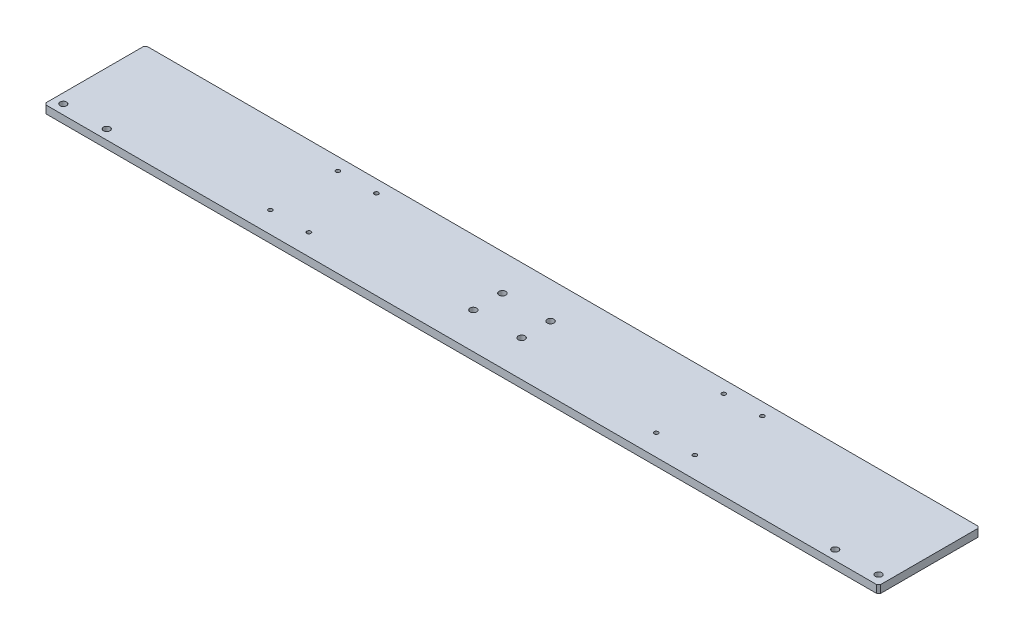
SolidWorks part; units mm, degrees
material "A6061"
ref_plane "前基準面" through (0, 0, 0) normal (0, 0, 1) x (1, 0, 0)
ref_plane "上基準面" through (0, 0, 0) normal (0, 1, 0) x (1, 0, 0)
ref_plane "右基準面" through (0, 0, 0) normal (1, 0, 0) x (0, 0, -1)
sketch "草图1" plane through (0, 0, 0) normal (0, 1, 0) x (1, 0, 0)
  line L1 (-432.5, -52.5) -> (432.5, -52.5)
  line L2 (-432.5, -52.5) -> (-432.5, 52.5)
  line L3 (-432.5, 52.5) -> (432.5, 52.5)
  line L4 (432.5, -52.5) -> (432.5, 52.5)
  line L5 (-432.5, -52.5) -> (432.5, 52.5) construction
  line L6 (-432.5, 52.5) -> (432.5, -52.5) construction
  point P0 (0, 0)
  dimension "D1" = 865
  dimension "D2" = 105
extrude "凸台-拉伸1" add sketch "草图1" along normal mid plane 8
chamfer "倒角1" distance 2 angle 45 4 edges at (432.5, 0, -52.5) (432.5, 0, 52.5) (-432.5, 0, -52.5) (-432.5, 0, 52.5)
hole_wizard "M5 螺纹孔1" positions "草图2" profile "草图3" tap size "M5" standard "GB" end condition through all
sketch "草图2" plane through (0, 4, 0) normal (0, 1, 0) x (1, 0, 0)
  line L0 (0, 107.0949) -> (0, 4.5) construction
  line L1 (0, 4.5) -> (-256.7344, 4.5) construction
  line L3 (430.5, 52.5) -> (-430.5, 52.5) construction
  point P0 (-220, 39.5)
  point P2 (-180, 39.5)
  point P10 (-180, -30.5)
  point P11 (-220, -30.5)
  point P12 (220, -30.5)
  point P13 (180, -30.5)
  point P14 (180, 39.5)
  point P15 (220, 39.5)
  dimension "D1" = 40
  dimension "D2" = 70
  dimension "D3" = 400
  dimension "D4" = 13
sketch "草图3" plane through (-220, 4, -39.5) normal (1, 0, 0) x (0, 0, 1)
  line L0 (0, 0) -> (0, 8)
  line L1 (0, 8) -> (2.1, 8)
  line L2 (2.1, 8) -> (2.1, 0)
  line L5 (2.1, 0) -> (0, 0)
  line L11 (0, -6.35) -> (0, 107.95) construction
  dimension "通孔螺纹孔钻头直径" = 4.2
  dimension "通孔螺纹孔钻头深度" = 8
cosmetic thread "孔螺蚊线1" parameters "D2"=5
cosmetic thread "孔螺蚊线2" parameters "D2"=5
cosmetic thread "孔螺蚊线3" parameters "D2"=5
cosmetic thread "孔螺蚊线4" parameters "D2"=5
cosmetic thread "孔螺蚊线5" parameters "D2"=5
cosmetic thread "孔螺蚊线6" parameters "D2"=5
cosmetic thread "孔螺蚊线7" parameters "D2"=5
cosmetic thread "孔螺蚊线8" parameters "D2"=5
hole_wizard "Ø7.0 (7) 直径孔1" positions "草图4" profile "草图5" hole size "Ø7.0" standard "GB" end condition through all
sketch "草图4" plane through (0, 4, 0) normal (0, 1, 0) x (1, 0, 0)
  line L0 (0, 81.503) -> (0, 0) construction
  line L1 (430.5, 52.5) -> (-430.5, 52.5) construction
  point P0 (25, -15)
  point P2 (25, 15)
  point P11 (-25, 15)
  point P12 (-25, -15)
  dimension "D1" = 50
  dimension "D2" = 30
  dimension "D3" = 37.5
sketch "草图5" plane through (25, 4, 15) normal (1, 0, 0) x (0, 0, 1)
  line L0 (0, 0) -> (0, 8)
  line L1 (0, 8) -> (3.5, 8)
  line L2 (3.5, 8) -> (3.5, 0)
  line L5 (3.5, 0) -> (0, 0)
  line L11 (0, -6.35) -> (0, 107.95) construction
  dimension "通孔孔直径" = 7
  dimension "通孔孔深度" = 8
hole_wizard "M8 螺纹孔1" positions "草图6" profile "草图7" tap size "M8" standard "GB" end condition through all
sketch "草图6" plane through (0, 4, 0) normal (0, 1, 0) x (1, 0, 0)
  line L0 (0, 0) -> (0, -71.3709) construction
  line L2 (-430.5, -52.5) -> (430.5, -52.5) construction
  line L5 (400, -30.5) -> (400, -59.1828) construction
  line L6 (-400, -30.5) -> (-400, -59.1828) construction
  point P0 (422.5, -42.5)
  point P2 (377.5, -42.5)
  point P8 (-377.5, -42.5)
  point P9 (-422.5, -42.5)
  dimension "D1" = 45
  dimension "D2" = 10
  dimension "D3" = 800
sketch "草图7" plane through (422.5, 4, 42.5) normal (1, 0, 0) x (0, 0, 1)
  line L0 (0, 0) -> (0, 8)
  line L1 (0, 8) -> (3.4, 8)
  line L2 (3.4, 8) -> (3.4, 0)
  line L5 (3.4, 0) -> (0, 0)
  line L11 (0, -6.35) -> (0, 107.95) construction
  dimension "通孔螺纹孔钻头直径" = 6.8
  dimension "通孔螺纹孔钻头深度" = 8
cosmetic thread "孔螺蚊线9" parameters "D2"=8
cosmetic thread "孔螺蚊线10" parameters "D2"=8
cosmetic thread "孔螺蚊线11" parameters "D2"=8
cosmetic thread "孔螺蚊线12" parameters "D2"=8
